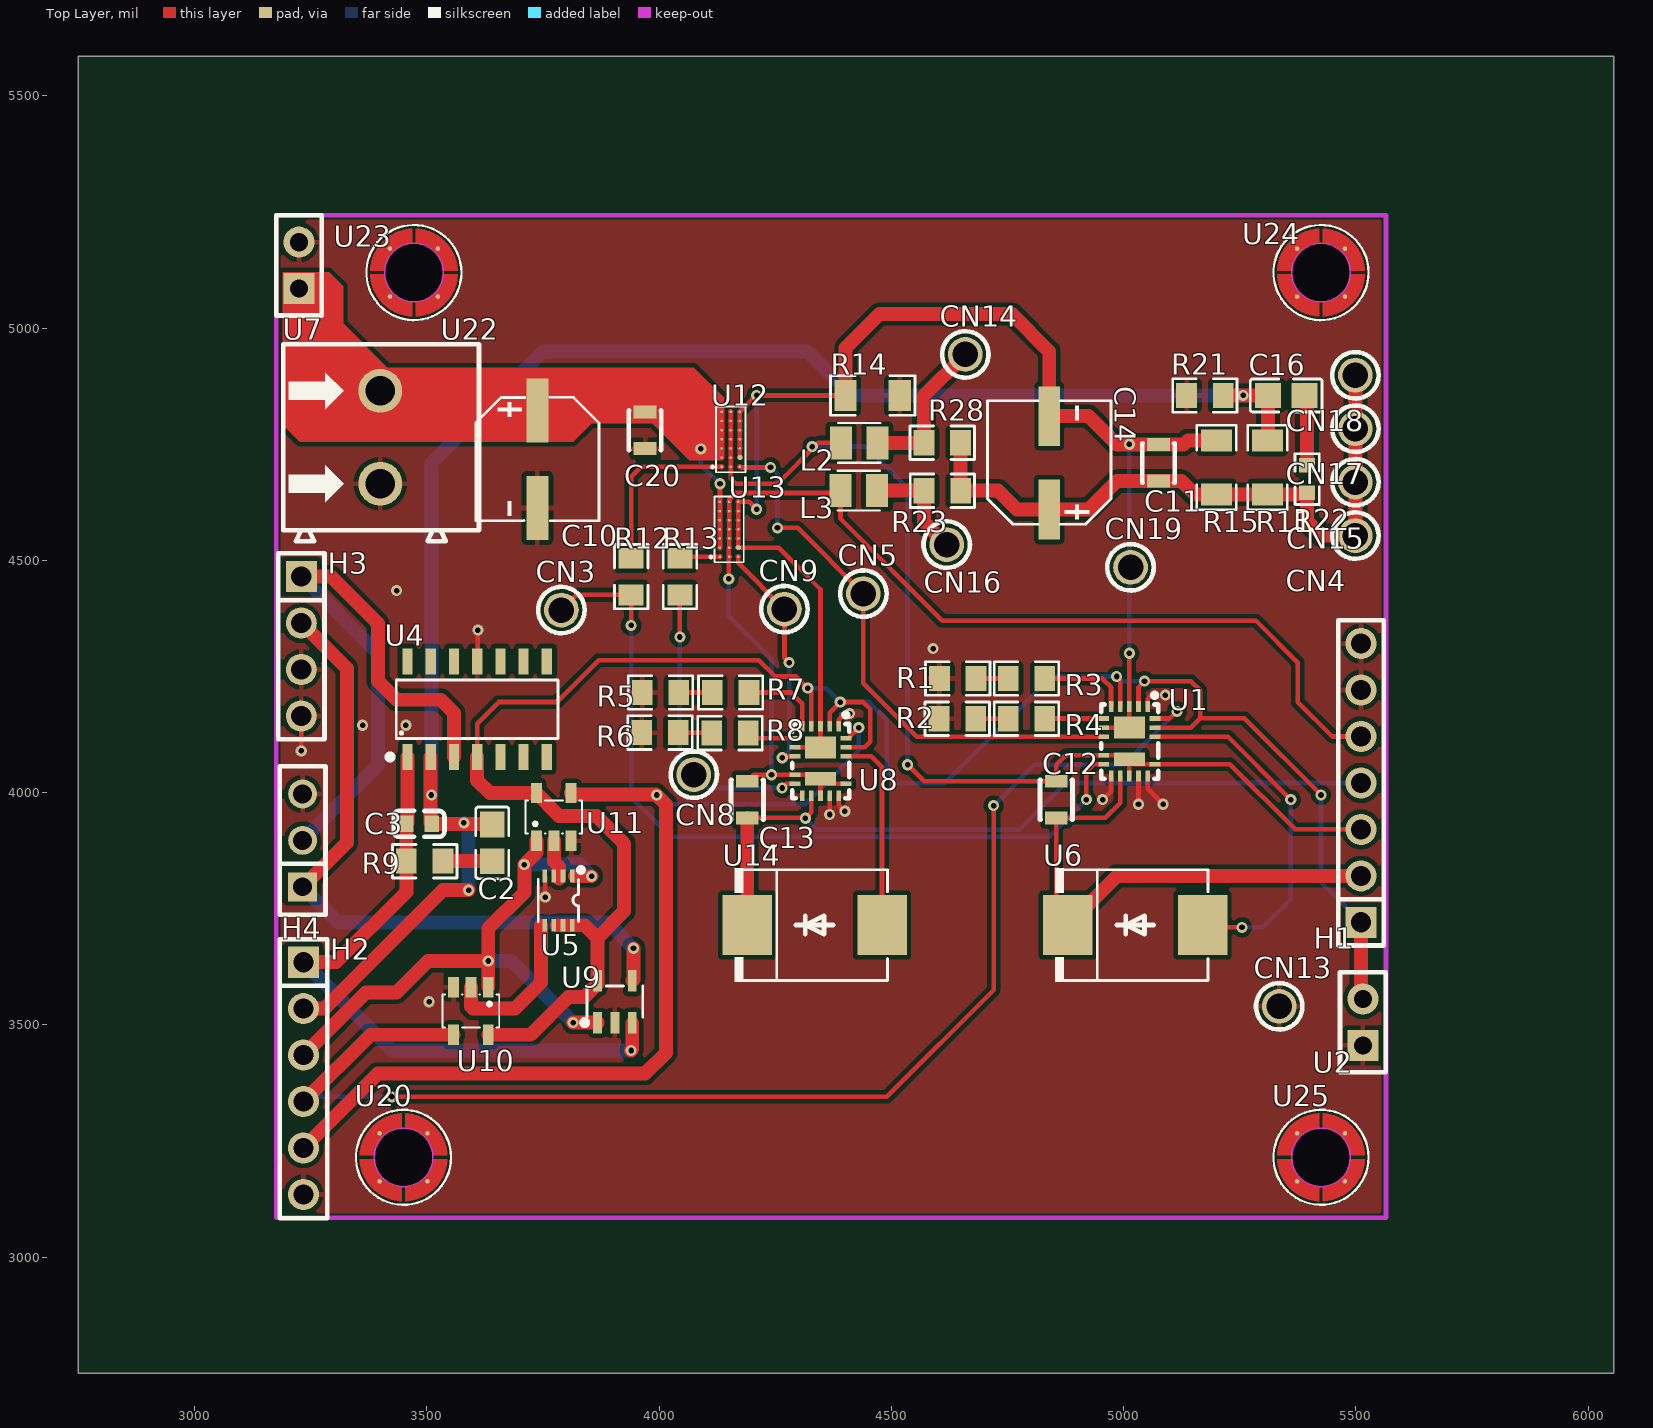
[diagram p0: Top Layer view]
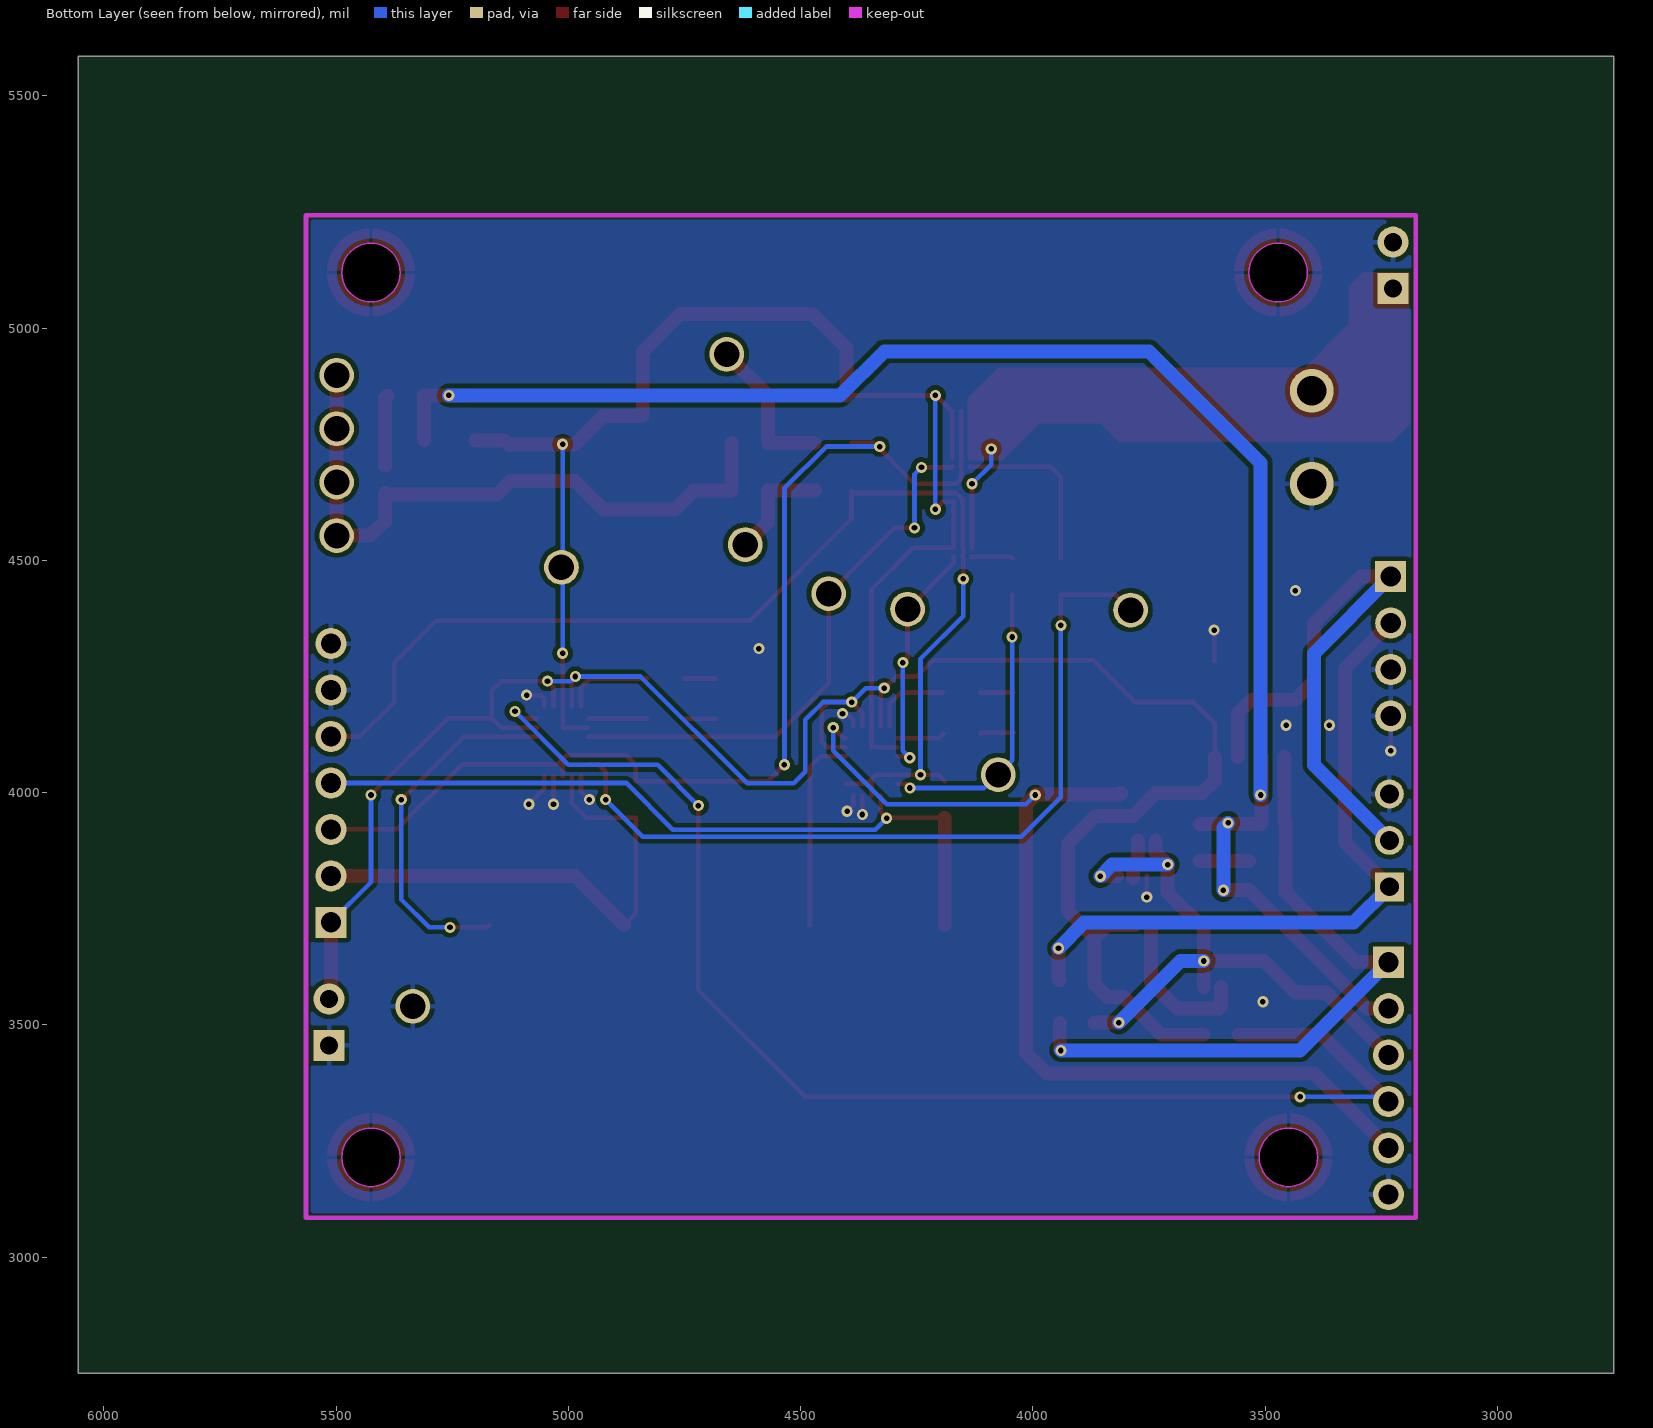
[diagram p1: Bottom Layer view, seen from below]
# Altium PCB MISC53275.pcbdoc
Units mil, origin at the board's own origin, x right, y up, seen from the top; angles counter-clockwise.
Board outline 3305 x 2835 mil, 2 copper layers (Top Layer, Bottom Layer), stack 62.206 mil thick; 63 components, 38 nets, 237 pads, 56 vias.

## Layer stack, top to bottom
Top Solder Mask Layer: solder mask 0.394, Dk 3.3
Top Layer: signal copper 1.379
Dielectric1: surface 59.449, FR4, Dk 4.5
Bottom Layer: signal copper 1.378
Bottom Solder Mask Layer: solder mask 0.394, Dk 3.3

## Board outline
6055,2750 2750,2750 2750,5585 6055,5585

## Design rules (kind name [scope] priority, off if disabled: settings)
BoardOutlineClearance copperThickness2oz_1 [All] p2 off: genericclearance=7.99 ignorepadtopadclearanceinfootprint=FALSE except(0: Arc-SplitContinuation Track-SplitContinuation SMDPad-SplitContinuation THPad-SplitContinuation Via-SplitContinuation Fill-SplitContinuation Region-SplitContinuation Poly-SplitContinuation Text-SplitContinuation Hole-SplitContinuation; 5.98: Arc-CutoutEdge SMDPad-CutoutEdge THPad-CutoutEdge Via-CutoutEdge Fill-CutoutEdge Region-CutoutEdge Text-CutoutEdge; 6.93: Hole-OutlineEdge Hole-CutoutEdge; 10: Poly-OutlineEdge Poly-CutoutEdge; 11.81: Arc-OutlineEdge Track-OutlineEdge SMDPad-OutlineEdge THPad-OutlineEdge Via-OutlineEdge Fill-OutlineEdge Region-OutlineEdge Text-OutlineEdge Track-CutoutEdge)
BoardOutlineClearance copperThickness1oz_1 [All] p4: genericclearance=4.02 ignorepadtopadclearanceinfootprint=FALSE except(0: SMDPad-CutoutEdge Arc-SplitContinuation Track-SplitContinuation SMDPad-SplitContinuation THPad-SplitContinuation Via-SplitContinuation Fill-SplitContinuation Region-SplitContinuation Poly-SplitContinuation Text-SplitContinuation Hole-SplitContinuation; 6: THPad-CutoutEdge Via-CutoutEdge Fill-CutoutEdge Region-CutoutEdge Text-CutoutEdge; 6.93: Hole-OutlineEdge Hole-CutoutEdge; 10: Poly-OutlineEdge Poly-CutoutEdge; 11.8: Arc-OutlineEdge Track-OutlineEdge SMDPad-OutlineEdge THPad-OutlineEdge Via-OutlineEdge Fill-OutlineEdge Region-OutlineEdge Text-OutlineEdge; 11.81: Arc-CutoutEdge Track-CutoutEdge)
Clearance copperThickness2oz [All] p1 off: gap=7.99 ignorepadtopadclearanceinfootprint=FALSE except(5.98: SMDPad-Track SMDPad-SMDPad THPad-Track SMDPad-THPad THPad-THPad Track-Via SMDPad-Via THPad-Via Via-Via Fill-Track Region-Track Fill-SMDPad Region-SMDPad Fill-THPad Region-THPad Fill-Via Region-Via Fill-Fill Fill-Region Region-Region Arc-Track Arc-SMDPad Arc-THPad Arc-Via Fill-Arc Region-Arc Arc-Arc Text-Track SMDPad-Text Text-THPad Text-Via Fill-Text Region-Text Arc-Text Text-Text; 6.93: Hole-Track Hole-SMDPad Hole-THPad Hole-Via Fill-Hole Region-Hole Hole-Arc Hole-Text; 10: Poly-Track Poly-SMDPad Poly-THPad Poly-Via Poly-Fill Poly-Region Poly-Poly Poly-Arc Poly-Text Poly-Hole)
Clearance copperThickness1oz [All] p3: gap=4.02 ignorepadtopadclearanceinfootprint=FALSE except(5.98: SMDPad-Track SMDPad-SMDPad THPad-Track SMDPad-THPad THPad-THPad Track-Via SMDPad-Via THPad-Via Via-Via Fill-Track Region-Track Fill-SMDPad Region-SMDPad Fill-THPad Region-THPad Fill-Via Region-Via Fill-Fill Fill-Region Region-Region; 6: Arc-Track Arc-SMDPad Arc-THPad Arc-Via Fill-Arc Region-Arc Arc-Arc Text-Track SMDPad-Text Text-THPad Text-Via Fill-Text Region-Text Arc-Text Text-Text; 6.93: Hole-Track Hole-SMDPad Hole-THPad Hole-Via Fill-Hole Region-Hole Hole-Arc Hole-Text; 10: Poly-Track Poly-SMDPad Poly-THPad Poly-Via Poly-Fill Poly-Region Poly-Poly Poly-Arc Poly-Text Poly-Hole)
DiffPairsRouting differentialPair [All] p1: maxlimit=6 minlimit=6 mostfreqgap=6 toplayer_minwidth=5 toplayer_prefwidth=10 toplayer_maxwidth=100 toplayer_mingap=6 toplayer_prefgap=6 toplayer_maxgap=6 bottomlayer_minwidth=5 bottomlayer_prefwidth=10 bottomlayer_maxwidth=100 bottomlayer_mingap=6 bottomlayer_prefgap=6 bottomlayer_maxgap=6 maxuncoupledlength=10
HoleToHoleClearance otherClearance [All] p1: gap=11.81 allowstackedmicrovias=TRUE
Length netLength [All] p1: minlimit=0 maxlimit=0
MatchedLengths netLengthTolerance [All] p1: tolerance=1000
PasteMaskExpansion pasteMaskExpansion [All] p1: expansion=0
PlaneConnect innerPlane [All] p1: planeconnectstyle=Relief reliefexpansion=20 reliefentries=4 reliefconductorwidth=10 reliefairgap=10
PolygonConnect copperRegion [(InNet('GND'))] p1: connectstyle=Relief reliefconductorwidth=10 reliefentries=4 polygonreliefangle="90 Angle" airgapwidth=10 via.connectstyle=Relief via.reliefconductorwidth=10 via.reliefentries=4 via.polygonreliefangle="90 Angle" via.airgapwidth=10
RoutingVias viaSize [All] p1: holewidth=12.01 width=24.02 viastyle="Through Hole" minholewidth=11.81 minwidth=19.68 maxholewidth=248.03 maxwidth=393.7
SolderMaskExpansion solderMaskExpansion [IsVia] p1: expansion=-1000 istentingtop=TRUE
SolderMaskExpansion solderMaskExpansion [All] p2: expansion=2 istentingtop=FALSE
Width copperThickness2oz_2 [All] p1 off: maxlimit=100 minlimit=8 preferedwidth=10
Width copperThickness1oz_2 [All] p2: maxlimit=100 minlimit=5 preferedwidth=10

## Components (designator, comment, footprint, x,y, rotation, side; value= is the part's Value field where it differs from the comment)
C2 "24pF" C0805 3641.16,3891.9 r90 top
C3 "0.6pF" C0603 3483.48,3932.7 r0 top
C10 "100uF" CAP-SMD_BD6.3-L6.6-W6.6-LS7.3-FD-H7.7 3738.19,4717.97 r270 top
C11 "100nF" CAP-SMD_L2.0-W1.25 5075,4710 r270 top
C12 "100nF" CAP-SMD_L2.0-W1.25 4855,3985 r270 top
C13 "100nF" CAP-SMD_L2.0-W1.25 4190,3985 r270 top
C14 "100uF" CAP-SMD_BD6.3-L6.6-W6.6-RD 4840,4710 r270 top
C16 "1.2pF" C0805 5350,4855 r0 top
C20 "100nF" CAP-SMD_L2.0-W1.25 3970,4780 r90 top
CN3 "RH-5001" TEST-TH_BD2.54-P1.4_BLACK 3789.9,4393.05 r0 top
CN4 "RH-5001" TEST-TH_BD2.54-P1.4_BLACK 5498.95,4553.36 r0 top
CN5 "RH-5001" TEST-TH_BD2.54-P1.4_BLACK 4439.9,4428.36 r0 top
CN8 "RH-5001" TEST-TH_BD2.54-P1.4_BLACK 4074.9,4038.68 r0 top
CN9 "RH-5001" TEST-TH_BD2.54-P1.4_BLACK 4270,4395 r0 top
CN13 "RH-5001" TEST-TH_BD2.54-P1.4_BLACK 5335,3540 r0 top
CN14 "RH-5001" TEST-TH_BD2.54-P1.4_BLACK 4659.27,4943.36 r0 top
CN15 "RH-5001" TEST-TH_BD2.54-P1.4_BLACK 5498.95,4668.36 r0 top
CN16 "RH-5001" TEST-TH_BD2.54-P1.4_BLACK 4619.27,4533.99 r0 top
CN17 "RH-5001" TEST-TH_BD2.54-P1.4_BLACK 5498.95,4783.36 r0 top
CN18 "RH-5001" TEST-TH_BD2.54-P1.4_BLACK 5498.95,4898.36 r0 top
CN19 "RH-5001" TEST-TH_BD2.54-P1.4_BLACK 5015,4485 r0 top
H1 "PZ254V-11-07P" HDR-TH_7P-P2.54-V-M 5511.17,4020.88 r90 top
H2 "PZ254V-11-06P" HDR-TH_6P-P2.54-V-M 3234.7,3385 r270 top
H3 "PZ254V-11-04P" HDR-TH_4P-P2.54-V-M 3230,4315 r270 top
H4 "PM254V-11-03-H85" HDR-TH_3P-P2.54-V-F 3232.73,3897.11 r90 top
L2 "100nH" IND-SMD_L2.3-W1.8 4430.77,4753.03 r0 top
L3 "100nH" IND-SMD_L2.3-W1.8 4430,4650 r0 top
R1 "120kΩ" R0805 4643.17,4245.58 r0 top
R2 "120kΩ" R0805 4642.17,4159.22 r0 top
R3 "20kΩ" R0805 4791.07,4245.58 r0 top
R4 "20kΩ" R0805 4791.07,4159.22 r0 top
R5 "120kΩ" R0805 4003.17,4215.58 r0 top
R6 "120kΩ" R0805 4002.17,4129.22 r0 top
R7 "20kΩ" R0805 4154.17,4215.58 r0 top
R8 "20kΩ" R0805 4152.66,4128.11 r0 top
R9 "100kΩ" R0805 3495.53,3852.53 r0 top
R11 "900kΩ" R1206 5310,4700 r270 top
R12 "4.7Ω" R0805 3940,4465 r90 top
R13 "4.7Ω" R0805 4045,4465 r90 top
R14 "0Ω" R1206 4460,4855 r180 top
R15 "600mΩ" R1206 5200,4700 r270 top
R21 "1.8MΩ" R0805 5175,4855 r0 top
R22 "69kΩ" R0603 5395,4675 r270 top
R23 "10mΩ" R0805 4610,4650 r0 top
R28 "10mΩ" R0805 4609.78,4753.03 r0 top
U1 "LMG1210RVRR" WQFN-19_L4.0-W3.0-P0.50-BL-EP_LMG1210RVRR 5012.44,4110.36 r270 top
U2 "ZX-PM2.54-1-2PY" HDR-TH_2P-P2.54-V-F 5515.17,3505.88 r90 top
U4 "AD8574ARZ-REEL7-HXY" SOP-14_L8.7-W3.9-P1.27-LS6.0-BL 3608.53,4179.64 r0 top
U5 "SN74LVC1G74DCUR" SSOP-8_L2.0-W2.3-P0.50-LS3.1-BR 3783.48,3767.7 r90 top
U6 "B540C" SMC_L6.9-W5.9-LS7.9-RD 5025,3715 r0 top
U7 "ZX-PM2.54-1-2PY" HDR-TH_2P-P2.54-V-F 3225,5135 r90 top
U8 "LMG1210RVRR" WQFN-19_L4.0-W3.0-P0.50-BL-EP_LMG1210RVRR 4347.66,4068.11 r270 top
U9 "LTC6752HS5#TRMPBF" SOT-23-5_L3.0-W1.7-P0.95-LS2.8-BL 3905,3550 r0 top
U10 "SN74LVC1G08DBVR" SOT-23-5_L3.0-W1.7-P0.95-LS2.8-BR 3595,3530 r90 top
U11 "SN74LVC1G08DBVR" SOT-23-5_L3.0-W1.7-P0.95-LS2.8-BR 3773.48,3947.7 r270 top
U12 "" 2111 4134.68,4701.57 r90 top
U13 "" 2111 4131.2,4507.74 r90 top
U14 "B540C" SMC_L6.9-W5.9-LS7.9-RD 4335,3715 r0 top
U20 "M3x10+6Cu" SMD_L4.7-W4.7-D3.0 3450,3215 r0 top
U22 "KF128-5.08-2P-AA" CONN-TH_P5.08_KF128-5.08-2P 3400,4765 r270 top
U23 "M3x10+6Cu" SMD_L4.7-W4.7-D3.0 3472.42,5119.51 r0 top
U24 "M3x10+6Cu" SMD_L4.7-W4.7-D3.0 5425,5119.51 r0 top
U25 "M3x10+6Cu" SMD_L4.7-W4.7-D3.0 5425,3215 r0 top

## Footprints (in the part's own frame and the unit in brackets; to place one, negate y for a bottom-side part, rotate by r counter-clockwise, add the part's x,y. Pads: shape width x height; smd on the part's side, far side on the other; paste and mask are expansions set on the pad)
2111 [mm]
  round 0.137 smd: 1(0,0) 2(0.5,0) 2(1,0) 2(1.5,0) 2(2,0) 2(2.5,0) 2(3,0) 3(0,-1) 4(1,-1) 4(1.5,-1) 4(2,-1) 4(2.5,-1) 4(3,-1) 5(0,-0.5) 5(0.5,-0.5) 5(1,-0.5) 5(1.5,-0.5) 5(2,-0.5) 5(2.5,-0.5) 5(3,-0.5)
  oct 0.275x0.276 smd: 4(0.5,-1)
  Top Layer region: -0.057,-0.362 0.056,-0.362 0.138,-0.443 0.138,-0.558 0.058,-0.638 -0.055,-0.638 -0.138,-0.556 -0.138,-0.443
  Top Layer region: -0.057,-0.862 0.056,-0.862 0.138,-0.943 0.138,-1.058 0.058,-1.138 -0.055,-1.138 -0.138,-1.056 -0.138,-0.943
  Top Layer region: -0.057,0.138 0.056,0.138 0.138,0.057 0.138,-0.058 0.058,-0.138 -0.055,-0.138 -0.138,-0.056 -0.138,0.057
  Top Layer region: 0.443,0.138 0.556,0.138 0.638,0.057 0.638,-0.058 0.558,-0.138 0.445,-0.138 0.362,-0.056 0.362,0.057
  Top Layer region: 0.443,-0.362 0.556,-0.362 0.638,-0.443 0.638,-0.558 0.558,-0.638 0.445,-0.638 0.362,-0.556 0.362,-0.443
  Top Layer region: 0.943,0.138 1.056,0.138 1.138,0.057 1.138,-0.058 1.058,-0.138 0.945,-0.138 0.862,-0.056 0.862,0.057
  Top Layer region: 0.943,-0.362 1.056,-0.362 1.138,-0.443 1.138,-0.558 1.058,-0.638 0.945,-0.638 0.862,-0.556 0.862,-0.443
  Top Layer region: 0.943,-0.862 1.056,-0.862 1.138,-0.943 1.138,-1.058 1.058,-1.138 0.945,-1.138 0.862,-1.056 0.862,-0.943
  Top Layer region: 1.443,0.138 1.556,0.138 1.638,0.057 1.638,-0.058 1.558,-0.138 1.445,-0.138 1.362,-0.056 1.362,0.057
  Top Layer region: 1.443,-0.862 1.556,-0.862 1.638,-0.943 1.638,-1.058 1.558,-1.138 1.445,-1.138 1.362,-1.056 1.362,-0.943
  Top Layer region: 1.443,-0.362 1.556,-0.362 1.638,-0.443 1.638,-0.558 1.558,-0.638 1.445,-0.638 1.362,-0.556 1.362,-0.443
  Top Layer region: 1.943,0.138 2.056,0.138 2.138,0.057 2.138,-0.058 2.058,-0.138 1.945,-0.138 1.862,-0.056 1.862,0.057
  Top Layer region: 1.943,-0.862 2.056,-0.862 2.138,-0.943 2.138,-1.058 2.058,-1.138 1.945,-1.138 1.862,-1.056 1.862,-0.943
  Top Layer region: 1.943,-0.362 2.056,-0.362 2.138,-0.443 2.138,-0.558 2.058,-0.638 1.945,-0.638 1.862,-0.556 1.862,-0.443
  Top Layer region: 2.443,0.138 2.556,0.138 2.638,0.057 2.638,-0.058 2.558,-0.138 2.445,-0.138 2.362,-0.056 2.362,0.057
  Top Layer region: 2.443,-0.862 2.556,-0.862 2.638,-0.943 2.638,-1.058 2.558,-1.138 2.445,-1.138 2.362,-1.056 2.362,-0.943
  Top Layer region: 2.443,-0.362 2.556,-0.362 2.638,-0.443 2.638,-0.558 2.558,-0.638 2.445,-0.638 2.362,-0.556 2.362,-0.443
  Top Layer region: 2.943,0.138 3.056,0.138 3.138,0.057 3.138,-0.058 3.058,-0.138 2.945,-0.138 2.862,-0.056 2.862,0.057
  Top Layer region: 2.943,-0.862 3.056,-0.862 3.138,-0.943 3.138,-1.058 3.058,-1.138 2.945,-1.138 2.862,-1.056 2.862,-0.943
  Top Layer region: 2.943,-0.362 3.056,-0.362 3.138,-0.443 3.138,-0.558 3.058,-0.638 2.945,-0.638 2.862,-0.556 2.862,-0.443
  silkscreen extent -0.3,-1.3 3.3,0.5
C0603 [mm]
  rect 0.8x0.9 smd: 1(-0.7,0) 2(0.7,0)
  silkscreen extent -1.39,-0.71 1.39,0.71
C0805 [mm]
  rect 1.41x1.35 smd paste-100 mask+0.051: 1(-1,0) 2(1,0)
  silkscreen extent -1.96,-0.9 1.96,0.9
CAP-SMD_BD6.3-L6.6-W6.6-LS7.3-FD-H7.7 [mm]
  rect 3.5x1.2 smd: 1(-2.67,0) 2(2.67,0)
  silkscreen extent -3.38,-3.38 3.38,3.38
CAP-SMD_BD6.3-L6.6-W6.6-RD [mm]
  rect 3.26x1.15 smd: 1(2.555,0) 2(-2.555,0)
  silkscreen extent -3.39,-3.38 3.36,3.38
CAP-SMD_L2.0-W1.25 [mm]
  rect 0.7x1.25 smd: 1(-1,0) 2(1,0)
  silkscreen extent -1.08,-0.89 1.08,0.89
CONN-TH_P5.08_KF128-5.08-2P [mm]
  round 2.4 hole 1.6: 1(-2.54,0) 2(2.54,0)
  silkscreen extent -5.08,-5.3 5.68,5.4
HDR-TH_2P-P2.54-V-F [mm]
  rect 1.7x1.7 hole 1: 1(-1.27,0)
  round 1.7 hole 1: 2(1.27,0)
  silkscreen extent -2.74,-1.25 2.74,1.25
HDR-TH_3P-P2.54-V-F [mil]
  rect 62x62 hole 40.16: 1(-100,0)
  round 62 hole 40.16: 2(0,0) 3(100,0)
  silkscreen extent -160,-49 160,49
HDR-TH_4P-P2.54-V-M [mm]
  rect 1.7x1.7 hole 1.1: 1(-3.81,0)
  round 1.7 hole 1.1: 2(-1.27,0) 3(1.27,0) 4(3.81,0)
  silkscreen extent -5.08,-1.27 5.08,1.27
HDR-TH_6P-P2.54-V-M [mm]
  rect 1.7x1.7 hole 1.1: 1(-6.35,0)
  round 1.7 hole 1.1: 2(-3.81,0) 3(-1.27,0) 4(1.27,0) 5(3.81,0) 6(6.35,0)
  silkscreen extent -7.6,-1.3 7.65,1.3
HDR-TH_7P-P2.54-V-M [mm]
  rect 1.7x1.7 hole 1.1: 1(-7.62,0)
  round 1.7 hole 1.1: 2(-5.08,0) 3(-2.54,0) 4(0,0) 5(2.54,0) 6(5.08,0) 7(7.62,0)
  silkscreen extent -8.89,-1.25 8.89,1.25
IND-SMD_L2.3-W1.8 [mm]
  rect 1.2x1.8 smd: 1(-1,0) 2(1,0)
  silkscreen extent -1.15,-1.09 1.15,1.09
R0603 [mil]
  rect 31.75x34.02 smd paste-3937.01 mask+2: 1(-29.66,0) 2(29.66,0)
  silkscreen extent -55,-26 55,26
R0805 [mm]
  rect 1.133x1.377 smd paste-100 mask+0.051: 1(-1,0) 2(1,0)
  silkscreen extent -1.76,-0.92 1.76,0.92
R1206 [mil]
  rect 47.54x66.97 smd paste-3937.01 mask+2: 1(-58.22,0) 2(58.22,0)
  silkscreen extent -91,-42 91,42
SMC_L6.9-W5.9-LS7.9-RD [mm]
  rect 2.7x3.3 smd: 1(-3.686,0) 2(3.686,0)
  silkscreen extent -4.36,-3.1 3.98,3.1
SMD_L4.7-W4.7-D3.0 [mm]
  round 0.249 smd: 1(-1.31,-1.31) 1(-1.31,1.31) 1(1.31,1.31) 1(1.31,-1.31)
  Top Layer region: 0.1,1.6 0.1,2.4 0.17,2.396 0.24,2.39 0.309,2.382 0.379,2.372 0.448,2.36 0.516,2.346 0.584,2.33 0.652,2.312 0.719,2.292 0.786,2.27 0.852,2.246 0.917,2.221 0.981,2.193 1.045,2.164 1.108,2.132 1.169,2.099 1.23,2.064 1.29,2.027 1.348,1.989 1.406,1.949 1.462,1.907 1.517,1.863 1.571,1.818 1.623,1.772 1.674,1.724 1.724,1.674 1.772,1.623 1.818,1.571 1.863,1.517 1.907,1.462 1.949,1.406 1.989,1.348 2.027,1.29 2.064,1.23 2.099,1.169 2.132,1.108 2.163,1.045 2.193,0.981 2.221,0.917 2.246,0.852 2.27,0.786 2.292,0.719 2.312,0.652 2.33,0.585 2.346,0.516 2.36,0.448 2.372,0.379 2.382,0.309 2.39,0.24 2.396,0.17 2.4,0.1 1.6,0.1 1.595,0.158 1.589,0.215 1.58,0.273 1.569,0.329 1.556,0.386 1.541,0.442 1.524,0.497 1.505,0.552 1.485,0.606 1.462,0.66 1.437,0.712 1.41,0.764 1.382,0.814 1.352,0.863 1.319,0.912 1.286,0.959 1.25,1.005 1.213,1.049 1.174,1.092 1.134,1.134 1.092,1.174 1.049,1.213 1.005,1.25 0.959,1.286 0.912,1.319 0.863,1.352 0.814,1.382 0.763,1.41 0.712,1.437 0.66,1.462 0.606,1.485 0.552,1.505 0.497,1.524 0.442,1.541 0.386,1.556 0.329,1.569 0.272,1.58 0.215,1.589 0.158,1.595
  Top Layer region: 1.6,-0.1 2.4,-0.1 2.396,-0.17 2.39,-0.24 2.382,-0.309 2.372,-0.379 2.36,-0.448 2.346,-0.516 2.33,-0.584 2.312,-0.652 2.292,-0.719 2.27,-0.786 2.246,-0.852 2.221,-0.917 2.193,-0.981 2.163,-1.045 2.132,-1.108 2.099,-1.169 2.064,-1.23 2.027,-1.29 1.989,-1.348 1.949,-1.406 1.907,-1.462 1.863,-1.517 1.818,-1.571 1.772,-1.623 1.724,-1.674 1.674,-1.724 1.623,-1.772 1.571,-1.818 1.517,-1.863 1.462,-1.907 1.406,-1.949 1.348,-1.989 1.29,-2.027 1.23,-2.064 1.169,-2.099 1.108,-2.132 1.045,-2.163 0.981,-2.193 0.917,-2.221 0.852,-2.246 0.786,-2.27 0.719,-2.292 0.652,-2.312 0.585,-2.33 0.516,-2.346 0.448,-2.36 0.379,-2.372 0.309,-2.382 0.24,-2.39 0.17,-2.396 0.1,-2.4 0.1,-1.6 0.158,-1.595 0.215,-1.589 0.272,-1.58 0.329,-1.569 0.386,-1.556 0.442,-1.541 0.497,-1.524 0.552,-1.505 0.606,-1.485 0.66,-1.462 0.712,-1.437 0.763,-1.41 0.814,-1.382 0.863,-1.351 0.912,-1.319 0.959,-1.286 1.005,-1.25 1.049,-1.213 1.092,-1.174 1.134,-1.134 1.174,-1.092 1.213,-1.049 1.25,-1.005 1.286,-0.959 1.319,-0.912 1.351,-0.863 1.382,-0.814 1.41,-0.763 1.437,-0.712 1.462,-0.66 1.484,-0.606 1.505,-0.552 1.524,-0.497 1.541,-0.442 1.556,-0.386 1.569,-0.329 1.58,-0.272 1.588,-0.215 1.595,-0.158
  Top Layer region: -0.1,-1.6 -0.1,-2.4 -0.17,-2.396 -0.24,-2.39 -0.309,-2.382 -0.379,-2.372 -0.448,-2.36 -0.516,-2.346 -0.584,-2.33 -0.652,-2.312 -0.719,-2.292 -0.786,-2.27 -0.852,-2.246 -0.917,-2.221 -0.981,-2.193 -1.045,-2.163 -1.108,-2.132 -1.169,-2.099 -1.23,-2.064 -1.29,-2.027 -1.348,-1.989 -1.406,-1.949 -1.462,-1.907 -1.517,-1.863 -1.571,-1.818 -1.623,-1.772 -1.674,-1.724 -1.724,-1.674 -1.772,-1.623 -1.818,-1.571 -1.863,-1.517 -1.907,-1.462 -1.949,-1.406 -1.989,-1.348 -2.027,-1.29 -2.064,-1.23 -2.099,-1.169 -2.132,-1.108 -2.163,-1.045 -2.193,-0.981 -2.221,-0.917 -2.246,-0.852 -2.27,-0.786 -2.292,-0.719 -2.312,-0.652 -2.33,-0.585 -2.346,-0.516 -2.36,-0.448 -2.372,-0.379 -2.382,-0.309 -2.39,-0.24 -2.396,-0.17 -2.4,-0.1 -1.6,-0.1 -1.595,-0.158 -1.589,-0.215 -1.58,-0.272 -1.569,-0.329 -1.556,-0.386 -1.541,-0.442 -1.524,-0.497 -1.505,-0.552 -1.485,-0.606 -1.462,-0.66 -1.437,-0.712 -1.41,-0.763 -1.382,-0.814 -1.352,-0.863 -1.319,-0.912 -1.286,-0.959 -1.25,-1.005 -1.213,-1.049 -1.174,-1.092 -1.134,-1.134 -1.092,-1.174 -1.049,-1.213 -1.005,-1.25 -0.959,-1.286 -0.912,-1.319 -0.863,-1.351 -0.814,-1.382 -0.763,-1.41 -0.712,-1.437 -0.66,-1.462 -0.606,-1.484 -0.552,-1.505 -0.497,-1.524 -0.442,-1.541 -0.386,-1.556 -0.329,-1.569 -0.272,-1.58 -0.215,-1.588 -0.158,-1.595
  Top Layer region: -1.599,0.1 -2.4,0.1 -2.396,0.17 -2.39,0.24 -2.382,0.309 -2.372,0.379 -2.36,0.448 -2.346,0.516 -2.33,0.585 -2.312,0.652 -2.292,0.72 -2.27,0.786 -2.246,0.852 -2.22,0.917 -2.193,0.982 -2.163,1.045 -2.132,1.108 -2.099,1.17 -2.064,1.23 -2.027,1.29 -1.988,1.348 -1.948,1.406 -1.906,1.462 -1.863,1.517 -1.818,1.571 -1.771,1.623 -1.723,1.674 -1.674,1.724 -1.623,1.772 -1.57,1.818 -1.517,1.863 -1.462,1.907 -1.405,1.949 -1.348,1.989 -1.289,2.027 -1.23,2.064 -1.169,2.099 -1.107,2.132 -1.045,2.164 -0.981,2.193 -0.917,2.221 -0.852,2.247 -0.786,2.27 -0.719,2.292 -0.652,2.312 -0.584,2.33 -0.516,2.346 -0.447,2.36 -0.378,2.372 -0.309,2.382 -0.239,2.39 -0.169,2.396 -0.099,2.4 -0.099,1.6 -0.157,1.595 -0.215,1.589 -0.272,1.58 -0.329,1.569 -0.386,1.556 -0.442,1.541 -0.497,1.524 -0.552,1.506 -0.606,1.485 -0.659,1.462 -0.712,1.437 -0.763,1.41 -0.814,1.382 -0.863,1.352 -0.911,1.32 -0.959,1.286 -1.004,1.25 -1.049,1.213 -1.092,1.174 -1.134,1.134 -1.174,1.092 -1.213,1.049 -1.25,1.005 -1.285,0.959 -1.319,0.912 -1.351,0.864 -1.381,0.814 -1.41,0.764 -1.437,0.712 -1.461,0.66 -1.484,0.606 -1.505,0.552 -1.524,0.498 -1.541,0.442 -1.556,0.386 -1.569,0.33 -1.579,0.273 -1.588,0.215 -1.595,0.158
  Board Outline Layer circle w0.003: c0,0 r1.6
  Board Outline Layer region: 1.6,0 1.442,-0.694 0.998,-1.251 0.356,-1.56 -0.356,-1.56 -0.998,-1.251 -1.442,-0.694 -1.6,0 -1.6,0 -1.442,0.694 -0.998,1.251 -0.356,1.56 0.356,1.56 0.998,1.251 1.442,0.694 1.6,0
  Board Outline Layer region: 1.6,0 1.59,-0.179 1.56,-0.356 1.51,-0.528 1.442,-0.694 1.355,-0.851 1.251,-0.998 1.131,-1.131 0.998,-1.251 0.851,-1.355 0.694,-1.442 0.528,-1.51 0.356,-1.56 0.179,-1.59 0,-1.6 -0.179,-1.59 -0.356,-1.56 -0.528,-1.51 -0.694,-1.442 -0.851,-1.355 -0.998,-1.251 -1.131,-1.131 -1.251,-0.998 -1.355,-0.851 -1.442,-0.694 -1.51,-0.528 -1.56,-0.356 -1.59,-0.179 -1.6,0 -1.59,0.179 -1.56,0.356 -1.51,0.528 -1.442,0.694 -1.355,0.851 -1.251,0.998 -1.131,1.131 -0.998,1.251 -0.851,1.355 -0.694,1.442 -0.528,1.51 -0.356,1.56 -0.179,1.59 0,1.6 0.179,1.59 0.356,1.56 0.528,1.51 0.694,1.442 0.851,1.355 0.998,1.251 1.131,1.131 1.251,0.998 1.355,0.851 1.442,0.694 1.51,0.528 1.56,0.356 1.59,0.179
  Multi-Layer board cut-out: 1.6,0 1.442,-0.694 0.998,-1.251 0.356,-1.56 -0.356,-1.56 -0.998,-1.251 -1.442,-0.694 -1.6,0 -1.6,0 -1.442,0.694 -0.998,1.251 -0.356,1.56 0.356,1.56 0.998,1.251 1.442,0.694 1.6,0
  silkscreen extent -2.6,-2.6 2.6,2.6
SOP-14_L8.7-W3.9-P1.27-LS6.0-BL [mm]
  rect 0.56x1.43 smd: 1(-3.81,-2.615) 2(-2.54,-2.615) 3(-1.27,-2.615) 4(0,-2.615) 5(1.27,-2.615) 6(2.54,-2.615) 7(3.81,-2.615) 8(3.81,2.615) 9(2.54,2.615) 10(1.27,2.615) 11(0,2.615) 12(-1.27,2.615) 13(-2.54,2.615) 14(-3.81,2.615)
  silkscreen extent -4.86,-2.71 4.43,1.6
SOT-23-5_L3.0-W1.7-P0.95-LS2.8-BL [mm]
  rect 0.49x1.157 smd: 1(-0.95,-1.154) 2(0,-1.154) 3(0.95,-1.154)
  rect 0.49x1.175 smd: 4(0.95,1.154) 5(-0.95,1.154)
  silkscreen extent -1.8,-1.29 1.53,0.85
SOT-23-5_L3.0-W1.7-P0.95-LS2.8-BR [mm]
  rect 1.1x0.6 smd: 1(1.3,-0.95) 2(1.3,0) 3(1.3,0.95) 4(-1.3,0.95) 5(-1.3,-0.95)
  silkscreen extent -0.9,-1.55 0.9,1.55
SSOP-8_L2.0-W2.3-P0.50-LS3.1-BR [mm]
  rect 0.7x0.26 smd: 1(1.35,-0.75) 2(1.35,-0.25) 3(1.35,0.25) 4(1.35,0.75) 5(-1.35,0.75) 6(-1.35,0.25) 7(-1.35,-0.25) 8(-1.35,-0.75)
  silkscreen extent -1.15,-1.37 1.81,1.1
TEST-TH_BD2.54-P1.4_BLACK [mm]
  round 1.9 hole 1.39: 1(0,0)
  silkscreen extent -1.27,-1.27 1.27,1.27
WQFN-19_L4.0-W3.0-P0.50-BL-EP_LMG1210RVRR [mm]
  rect 0.6x0.25 smd paste+0 mask+0.05: 1(-1.9,1) 2(-1.9,0.5) 3(-1.9,0) 4(-1.9,-0.5) 5(-1.9,-1) 11(1.9,-1) 12(1.9,-0.5) 13(1.9,0) 14(1.9,0.5) 15(1.9,1)
  rect 0.25x0.6 smd paste+0 mask+0.05: 6(-1.25,-1.4) 7(-0.75,-1.4) 8(-0.25,-1.4) 9(0.75,-1.4) 10(1.25,-1.4) 16(1.25,1.4) 17(-0.25,1.4) 18(-0.75,1.4) 19(-1.25,1.4)
  rect 1.2x1.7 smd paste+0 mask+0.05: 20(-0.75,0)
  rect 0.75x1.7 smd paste+0 mask+0.05: 21(0.975,0)
  silkscreen extent -2.65,-1.54 2.04,1.58

## Via types
v1: diameter 24.02, hole 12, Top Layer to Bottom Layer, 56 vias

## Nets (pads, with @x,y where several pads share a name; then routed paths per layer and width w, separated by ;. In a path a pad name is that pad's centre, name@x,y a point inside that pad or via, vN(x,y) a via of type N, cw(c..) or ccw(c..) an arc to the next point about the centre after c; other vN are vias at no path point)
$1N43: C16.2 R22.1 | length 152.7
  Top Layer w30: C16.2 5395,4849.37 R22.1
$1N51: R13.2 U13.1 | length 87.6
  Top Layer w10: R13.2 4048.37,4507.74 U13.1@4131.2,4507.74
$1N54: R12.2 U12.1 | length 379.3
  Top Layer w10: R12.2 3940,4680 3961.57,4701.57 U12.1
$1N71: C2.1 R9.2 | length 106.3
  Top Layer w30: R9.2 C2.1
$1N89: R6.2 R8.1 | length 72.2
  Top Layer w10: R6.2 4112.18,4129.22 R8.1
$1N91: R8.2 U8.6 | length 105
  Top Layer w10: R8.2 4202.81,4117.33 U8.6
$1N92: R5.2 R7.1 | length 72.3
  Top Layer w10: R5.2 R7.1
$1N93: R7.2 U8.5 | length 173.4
  Top Layer w10: R7.2 4284.42,4215.58 4308.28,4191.72 U8.5
$1N112: R2.2 R4.1 | length 70.2
  Top Layer w10: R2.2 R4.1
$1N114: R4.2 U1.6 | length 127
  Top Layer w10: R4.2 4830.79,4159.57 U1.6
$1N115: R1.2 R3.1 | length 69.2
  Top Layer w10: R1.2 R3.1
$1N116: R3.2 U1.5 | length 192.1
  Top Layer w10: R3.2 4954.42,4245.58 4973.06,4226.94 U1.5
BST1: U1.17 U6.2 | length 780.2
  Top Layer w10: U1.17 5224.8,4120.2 v1(5360,3985) ; U6.2 5175.13,3710 v1(5255,3710)
  Bottom Layer w10: v1(5255,3710) 5300,3710 5360,3770 v1(5360,3985)
BST2: U8.17 U14.2 | length 426.8
  Top Layer w10: U8.17 4457.04,4077.96 4480.13,4054.87 U14.2
CLK1: U5.5 U10.2 | length 341
  Top Layer w30: U10.2 3595,3540 3600,3535 3690,3535 3746.03,3591.03 3746.03,3714.55
CLK2: U5.2 U5.3 U11.2 | length 86.3
  Top Layer w30: U11.2 3773.48,3851.52 3785,3840 3785,3815
FB: C2.2 C3.2 C16.1 H2.2 R11.1 R21.2 U4.2 | length 3680.2
  Top Layer w30: H2.2 3280,3535 3535,3790 v1(3590,3790) ; U4.2 3508.53,3935.21 C3.2 3639.72,3932.7 C2.2 ; R21.2 v1(5257.3,4855) C16.1 5310.63,4758.85 R11.1
  Bottom Layer w30: v1(3510,3995) 3510,4710 3750,4950 4320,4950 4415,4855 v1(5257.3,4855) ; v1(3580,3935) 3590,3925 v1(3590,3790)
GND: C10.2 C20.1 CN13.1 H1.6 H1.7 H2.6 H3.3 H3.4 H4.3 R1.1 R2.1 R5.1 R6.1 R14.1 R21.1 U1.1 U1.11 U1.14 U1.15 U2.1 U4.11 U5.4 U7.2 U8.1 U8.11 U8.14 U8.15 U9.2 U10.3 U11.3 U22.2 | length 561.9
  Top Layer w10: v1(3230,4090) H3.4 ; U4.11 3610,4284.07 v1(3610,4350) ; U5.4 3755,3819.79 v1(3755,3775) ; v1(4367.34,3952.99) U8.14 ; U8.15 4387.02,3972.98 v1(4400,3960) ; U8.1 4387.02,4157.02 4400,4170 v1(4410,4170) ; v1(4955,3985) 4973.06,4003.06 U1.11 ; v1(5032.12,3975) U1.14 ; U1.15 5051.8,4008.2 v1(5085,3975) ; U1.1 5051.8,4201.8 5060,4210 v1(5090,4210)
  other v1: 3505,3550 3361.98,4145 3455,4145 4590,4310 3435,4435
HB1: C12.2 H1.2 U1.12 U6.1 | length 1124.9
  Top Layer w10: U6.1 4855,3739.87 C12.2 4960.63,3945.63 4992.75,3977.75 U1.12
  Top Layer w30: U6.1 4985.75,3820.88 H1.2
HB2: C13.2 H1.4 U8.12 U14.1 | length 1657.4
  Top Layer w10: C13.2 4315.63,3945.63 4327.97,3957.97 U8.12
  Top Layer w30: U14.1 4189.87,3945.5 C13.2
  Bottom Layer w10: v1(4315,3945) 4340,3920 4775,3920 4875.88,4020.88 H1.4
HO1: CN3.1 R12.1 U1.10 | length 1751.6
  Top Layer w10: CN3.1 3822.48,4425.63 R12.1 v1(3940,4360) ; v1(4920,3985) 4920,4045 4936.14,4061.14 U1.10
  Bottom Layer w10: v1(3940,4360) 3940,3990 4025,3905 4840,3905 v1(4920,3985)
HO2: CN8.1 R13.1 U8.10 | length 631.7
  Top Layer w10: v1(4045,4335) R13.1 ; v1(4265,4010) 4273.9,4018.9 U8.10
  Bottom Layer w10: v1(4045,4335) 4045,4070 4105,4010 v1(4265,4010)
HS1: C12.1 H1.3 L2.1 U1.9 U1.13 U1.16 U1.21 U12.5 | length 2397.1
  Top Layer w10: U12.5@4154.37,4819.68 4154.37,4800 4154.37,4780.31 4154.37,4760.63 4154.37,4740.95 4154.37,4721.26 4154.37,4701.57 4154.37,4675.63 4165,4665 4255,4665 4343.03,4753.03 L2.1 ; v1(4535,4060) 4570.63,4024.37 C12.1 4855,4060 4875.83,4080.83 U1.9 5003.57,4080.83 U1.21 ; U1.13 U1.21 ; H1.3 5369.12,3920.88 5228.86,4061.14 U1.16 5023.26,4061.14 U1.21
  Bottom Layer w10: v1(4330,4745) 4445,4745 4535,4655 v1(4535,4060)
HS2: C13.1 H1.5 L3.1 U8.9 U8.13 U8.16 U8.21 U13.5 | length 2566.7
  Top Layer w10: v1(4150,4460) 4150,4526.54 4150.89,4527.43 4150.89,4547.12 4150.89,4566.8 4150.89,4586.48 4150.89,4606.17 4150.89,4625.85 4150.89,4630.89 4165,4645 4385.63,4645 L3.1 4390.63,4589.37 4610,4370 5285,4370 5375,4280 5375,4195 5449.12,4120.88 H1.5 ; C13.1 4204.22,4038.59 v1(4242.12,4038.59) U8.9 4338.79,4038.59 U8.21 ; U8.13 U8.21 ; U8.16 4358.48,4018.9 U8.21
  Bottom Layer w10: v1(4150,4460) 4150,4380 4242.12,4287.88 v1(4242.12,4038.59)
IL1+: CN14.1 L2.2 R28.1 | length 327.4
  Top Layer w30: L2.2 R28.1 4570.41,4854.51 CN14.1
IL1-: C11.2 C14.1 CN4.1 CN15.1 CN17.1 CN18.1 R11.2 R15.2 R22.2 R23.2 R28.2 | length 1426.7
  Top Layer w30: R28.2 4649.37,4752.81 R23.2 4730,4650 4770.59,4609.41 C14.1 4924.41,4609.41 4985.63,4670.63 C11.2 5124.37,4670.63 5153.22,4641.78 R15.2 R11.2 5391.44,4641.78 R22.2 5395,4585 5426.64,4553.36 CN4.1 CN15.1 CN17.1 CN18.1
IL2+: CN16.1 L3.2 R23.1 | length 237.4
  Top Layer w30: L3.2 R23.1 4570.63,4582.63 CN16.1
IR2-: C11.1 C14.2 CN19.1 R14.2 R15.1 U1.3 U1.7 U1.20 U8.3 U8.7 U8.20 U12.4 U13.4 | length 3136.5
  Top Layer w10: U12.4@4174.06,4721.26 4174.06,4740.94 4174.06,4760.63 4174.06,4780.31 4174.06,4800 4174.06,4819.68 4209.37,4855 R14.2 ; v1(4210,4610) 4194.15,4625.85 4170.57,4625.85 4170.57,4606.17 4170.57,4586.48 4170.57,4566.8 4170.57,4547.12 4170.57,4527.43 4257.57,4527.43 4347.65,4437.35 U8.3 U8.20 U8.7 ; U1.7 U1.20 U1.3 v1(5012.43,4300)
  Top Layer w30: R14.2 4401.78,4956.78 4475,5030 4760,5030 4840,4950 C14.2 4924.41,4810.59 4985.63,4749.37 C11.1 5129.37,4749.37 5138.22,4758.22 R15.1
  Bottom Layer w10: v1(4210,4610) v1(4210,4855) ; v1(5012.43,4300) v1(5012.43,4750)
LO1: CN5.1 U1.8 U12.3 | length 1204.7
  Top Layer w10: U12.3 4175.63,4700 v1(4240,4700) ; v1(4255,4570) 4298.26,4570 CN5.1 4439.9,4235.1 4554.8,4120.2 U1.8
  Bottom Layer w10: v1(4240,4700) 4255,4685 v1(4255,4570)
LO2: CN9.1 U8.8 U13.3 | length 512.9
  Top Layer w10: U13.3@4170.57,4507.74 4170.57,4494.43 CN9.1 4270,4290 v1(4280,4280) ; v1(4265.11,4075) 4268.07,4077.96 U8.8
  Bottom Layer w10: v1(4265.11,4075) 4280,4089.89 v1(4280,4280)
PWL: H3.2 H4.1 U9.4 | length 1485.6
  Top Layer w30: H3.2 3327.99,4267.01 3327.99,3892.37 H4.1 ; U9.4 3945,3598.02 v1(3945,3665)
  Bottom Layer w30: H4.1 3309.84,3720 3890,3720 v1(3945,3665)
PWM: H2.3 U5.1 U9.1 U10.1 U11.1 | length 1321.5
  Top Layer w30: H2.3 3369.7,3570 3435,3570 3502.64,3637.64 v1(3632.4,3637.64) ; U10.1 v1(3632.4,3637.64) ; U11.1 3736.08,3871.08 v1(3710,3845) 3710,3785 3632.4,3707.4 v1(3632.4,3637.64) ; v1(3815,3505) 3867.18,3505 U9.1 ; 3819.42,3820.85 3820.26,3820 v1(3855,3820)
  Bottom Layer w30: v1(3632.4,3637.64) 3682.36,3637.64 v1(3815,3505) ; v1(3710,3845) 3830,3845 v1(3855,3820)
PWM1: H2.4 U1.19 U10.4 | length 2897
  Top Layer w10: v1(3425,3345) 4490,3345 4720.18,3575.18 v1(4720.18,3972.03) ; U1.19 5099.57,4159.57 v1(5115,4175)
  Top Layer w30: H2.4 3378.51,3478.82 U10.4
  Bottom Layer w10: H2.4 3244.7,3345 v1(3425,3345) ; v1(4720.18,3972.03) 4808.15,4060 5000,4060 v1(5115,4175)
PWM2: H2.5 U8.19 U11.4 | length 2191.8
  Top Layer w10: U8.19 4407.33,4117.33 v1(4430,4140)
  Top Layer w30: H2.5 3394.7,3395 3970,3395 4015,3440 4015,3975 3993.79,3996.21 3813.55,3996.21 U11.4
  Bottom Layer w10: v1(3995,3995) 4015,3975 4315,3975 4430,4090 v1(4430,4140)
VDD: H1.1 U1.2 U1.4 U1.18 U2.2 U4.4 U5.6 U5.7 U5.8 U8.2 U8.4 U8.18 U9.5 U10.5 U11.5 | length 4540.6
  Top Layer w10: U4.4 3608.53,4148.53 3655,4195 3780,4195 3870,4285 4215,4285 4250,4250 4295,4250 v1(4320,4225) 4327.97,4217.03 U8.4 ; U8.2 4367.34,4172.34 v1(4390,4195) 4440,4195 4455,4180 4455,4110 4442.64,4097.64 U8.18 ; v1(4985,4250) 4992.75,4242.25 U1.4 ; U1.2 5032.12,4227.12 v1(5045,4240) 5145,4240 5165,4220 5165,4160 ; U1.18 5144.88,4139.88 5165,4160 ; v1(5425,3995) 5260,4160 5165,4160
  Top Layer w30: U4.4 3608.53,4026.47 3636.11,3998.89 U11.5 3784.96,3950 3865,3950 3925,3890 3925,3744.8 3867.6,3687.4 ; U10.5 3723.82,3478.82 3805,3560 3840,3560 3867.6,3587.6 U9.5 3867.6,3687.4 ; 3780.05,3714.55 U5.7 U5.8 3840.45,3714.55 3867.6,3687.4 ; H1.1 5511.17,3559.88 U2.2
  Bottom Layer w10: v1(4320,4225) 4360,4225 v1(4390,4195) 4452.03,4195 4490,4157.03 4490,4045 4515,4020 4615,4020 4845,4250 v1(4985,4250) 4995,4240 v1(5045,4240) ; v1(5425,3995) 5425,3807.05 H1.1
VE: C3.1 H2.1 R9.1 U4.1 U9.3 | length 1420.4
  Top Layer w30: H2.1 3305,3635 3456.16,3786.16 R9.1 3455.92,3852.77 C3.1 3458.53,3935.31 U4.1 ; v1(3940,3445) 3942.4,3447.4 U9.3
  Bottom Layer w30: H2.1 3424.7,3445 v1(3940,3445)
VIN: C10.1 C20.2 U7.1 U12.2 U13.2 U22.1 | length 229.6
  Top Layer w10: U13.2@4131.2,4527.43 4131.2,4547.12 4131.2,4566.8 4131.2,4586.48 4131.2,4606.17 4131.2,4625.85 v1(4131.2,4665)
  Bottom Layer w10: v1(4090,4740) 4090,4706.2 v1(4131.2,4665)
VREF: H3.1 H4.2 U4.3 | length 1320.9
  Top Layer w30: H3.1 3293.79,4465 3395,4363.79 3395,4240 3435,4200 3530,4200 3558.53,4171.47 U4.3
  Bottom Layer w30: H3.1 3395,4300 3395,4059.38 H4.2
pads on no net: U4.5 U4.6 U4.7 U4.8 U4.9 U4.10 U4.12 U4.13 U4.14 U20.1 U23.1 U24.1 U25.1

## Polygon pours and split planes (outlines as drawn)
GND on Top Layer (solid, remove dead copper, pour order 0): 3000,5335 3000,3000 5805,3000 5805,5335
GND on Bottom Layer (solid, remove dead copper, pour order 2): 3055,5320 3055,3010 5645,3010 5645,5320

## Keep-outs
Board Outline Layer:
  lines w10: 3175.79,3085 3175.79,5242.87 5565,5242.87 5565,3085 3175.79,3085

## Other copper
Top Layer:
  region net VIN: 3190,5120 3290,5120 3320,5090 3320,5010.28 3415.28,4915 4075,4915 4140,4850 4140,4720 4135,4715 4065,4715 3985,4795 3855,4795 3815,4755 3226.6,4755 3190,4791.6